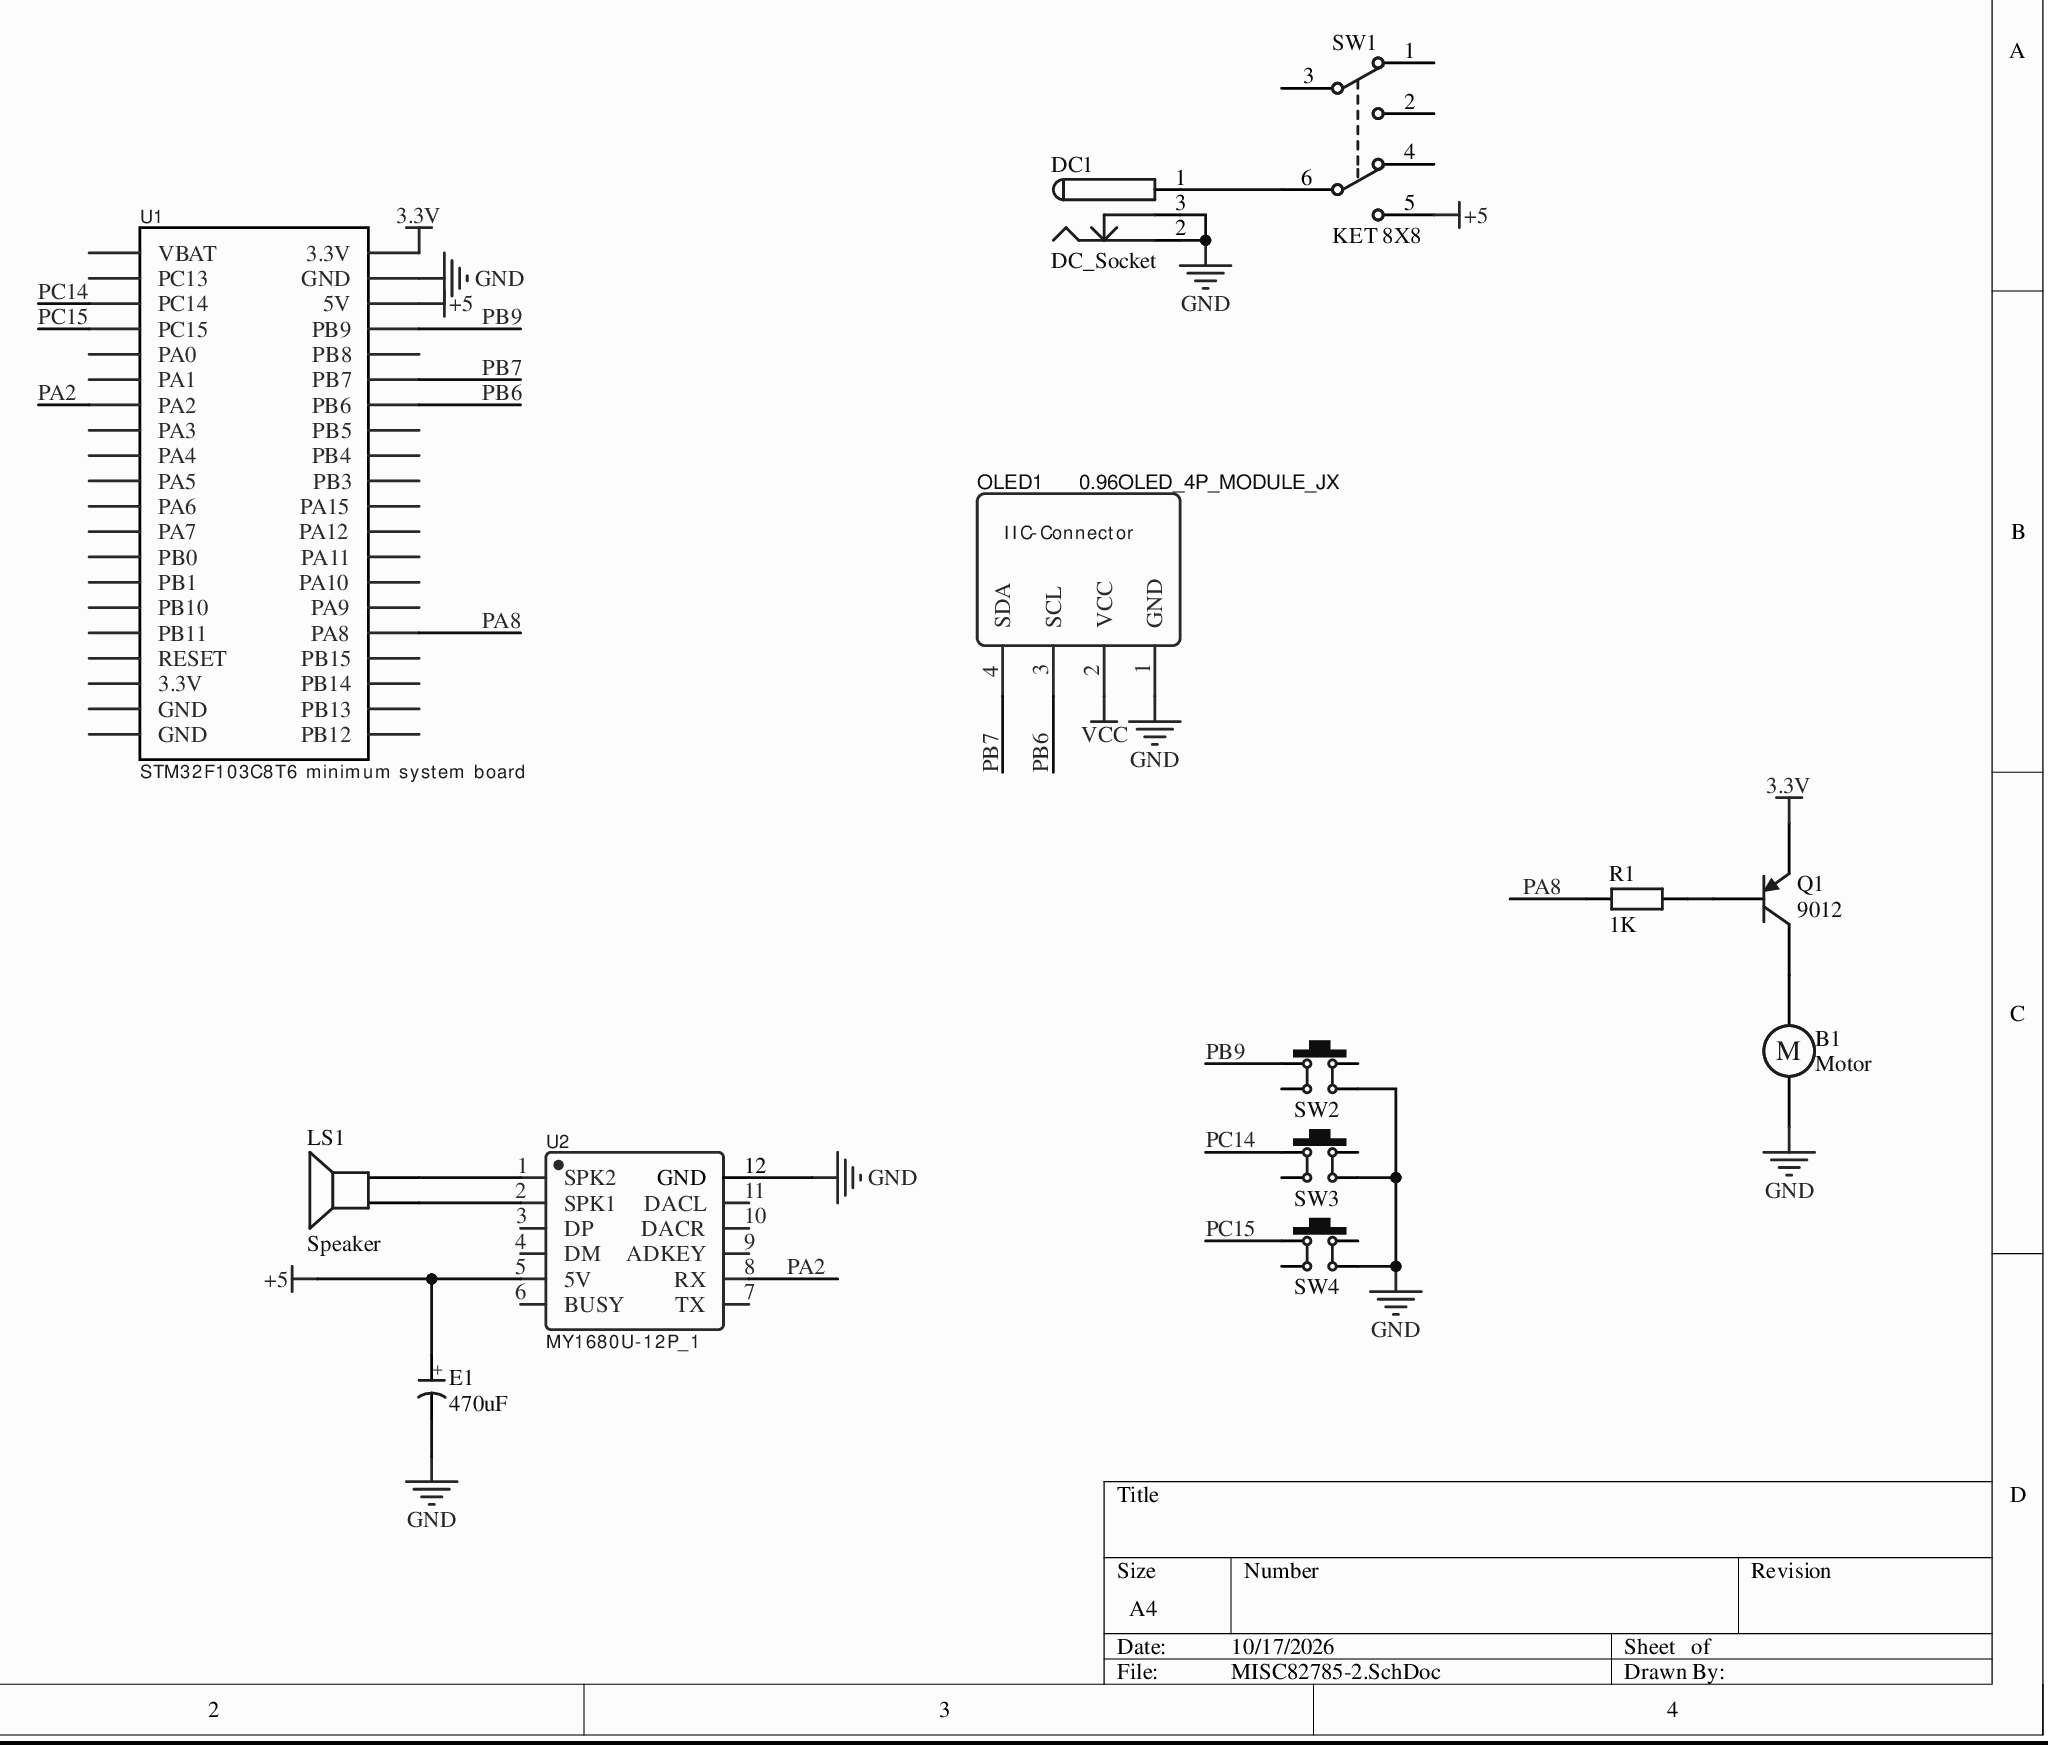
[diagram p0: MISC82785-2.SchDoc]
# Altium project MISC82785-6.PrjPcb
1 sheet, 13 parts. Net scope: global (net labels, ports and power ports of the same name join across sheets).
Board file: MISC82785.PcbDoc

## Sheet MISC82785-2.SchDoc
size A4

### Parts
B1  Motor  [RB5-10.5]
DC1  DC_Socket  [DC-002]
E1  470uF  [CS 2.0*5*8 - C]
LS1  Speaker  [PIN2]
OLED1  0.96OLED_4P_MODULE_JX  [0.96OLED_4P]
Q1  9012  [TO-92A]
R1  1K  [RS 1/4W]
SW1  KET 8X8  [KFT DIP-8X8]
SW2  6x6x5  [TSW DIP-6*6*6]  (value not drawn)
SW3  6x6x5  [TSW DIP-6*6*6]  (value not drawn)
SW4  6x6x5  [TSW DIP-6*6*6]  (value not drawn)
U1  STM32F103C8T6 minimum system board  [STM32核心板]
U2  MY1680U-12P_1  [COMM-TH_MY1680-12P]

### Nets
3.3V: Q1.1(E) U1.40(3.3V)
+5: E1.1(A) SW1.5(COM2) U1.38(5V) U2.5(5V)
GND: B1.2 DC1.2 DC1.3 E1.2(K) OLED1.1(GND) SW2.3 SW3.3 SW4.3 U1.39(GND) U2.12(GND)
VCC: OLED1.2(VCC)
PA2: U1.7(PA2) U2.8(RX)
PA8: R1.1 U1.25(PA8)
PB6: OLED1.3(SCL) U1.34(PB6)
PB7: OLED1.4(SDA) U1.35(PB7)
PB9: SW2.1 U1.37(PB9)
PC14: SW3.1 U1.3(PC14)
PC15: SW4.1 U1.4(PC15)
NetB1_1: B1.1 Q1.3(C)
NetDC1_1: DC1.1 SW1.6(NC2)
NetLS1_1: LS1.1 U2.2(SPK1)
NetLS1_2: LS1.2 U2.1(SPK2)
NetQ1_2: Q1.2(B) R1.2

Not connected (* = marked no-connect by the designer): SW1 1(NC1) 2(COM2) 3(NO1) 4(NO2); SW2 2 4; SW3 2 4; SW4 2 4; U1 1(VBAT) 2(PC13) 5(PA0) 6(PA1) 8(PA3) 9(PA4) 10(PA5) 11(PA6) 12(PA7) 13(PB0) 14(PB1) 15(PB10) 16(PB11) 17(RESET) 18(3.3V) 19(GND) 20(GND) 21(PB12) 22(PB13) 23(PB14) 24(PB15) 26(PA9) 27(PA10) 28(PA11) 29(PA12) 30(PA15) 31(PB3) 32(PB4) 33(PB5) 36(PB8); U2 3(DP) 4(DM) 6(BUSY) 7(TX) 9(ADKEY) 10(DACR) 11(DACL)

### Library data of the parts
B1 = Motor: Motor, General Kind; Published: 24-Mar-1999; LatestRevisionDate: 17-Jul-2002; LatestRevisionNote: Re-released for DXP Platform.; PackageReference: RB5-10.5; PackageDescription: Capacitor (Radial); 2 Leads; Publisher: Altium Limited
E1 = CS: THT solid capacitor; BOM名称: THT solid capacitor
LS1 = Speaker: Loudspeaker; Published: 24-Mar-1999; LatestRevisionDate: 17-Jul-2002; LatestRevisionNote: Re-released for DXP Platform.; PackageReference: PIN2; Publisher: Altium Limited
OLED1 = 0.96OLED_4P_MODULE_JX: Manufacturer: null; Contributor: LCSC; Supplier: LCSC; Supplier Part: C9900004566; Manufacturer Part: 0.96OLED_4P_MODULE_JX; JLCPCB Part Class: Extended Part; link: https://so.szlcsc.com/global.html?k=C9900004566&ref=editor; spicePre: O; spiceSymbolName: 0.96OLED_4P_MODULE_JX
Q1 = 2N3906: PNP General Purpose Amplifier; Published: 8-Jun-2000; LatestRevisionDate: 15-Jan-2003; LatestRevisionNote: PCB Footprint 'BCY-W3/D4.7' replaced; DatasheetVersion: 1997; PackageVersion: Sep-1998; PackageReference: TO-92A; PackageDescription: TO, Flat Index; 3 In-Line, Axial Leads; Body Dia. 4.5mm; Leads 0.51 x 0.48 mm (max); ComponentLink1Description: Manufacturer Link; ComponentLink2Description: Datasheet; ComponentLink2URL: http://www.fairchildsemi.com/ds/2N%2F2N3906.pdf; Publisher: Altium Limited
R1 = R-S: Color-band resistor; BOM名称: Color-band resistor
SW1 = KET 8X8: 8*8 self-locking switch; BOM名称: 8*8 self-locking switch
SW2-SW4 = TSW DIP-6x6: THT 6x6 tactile switch; BOM名称: THT 6x6 tactile switch
U1 = STM32F103C8T6最小系统板